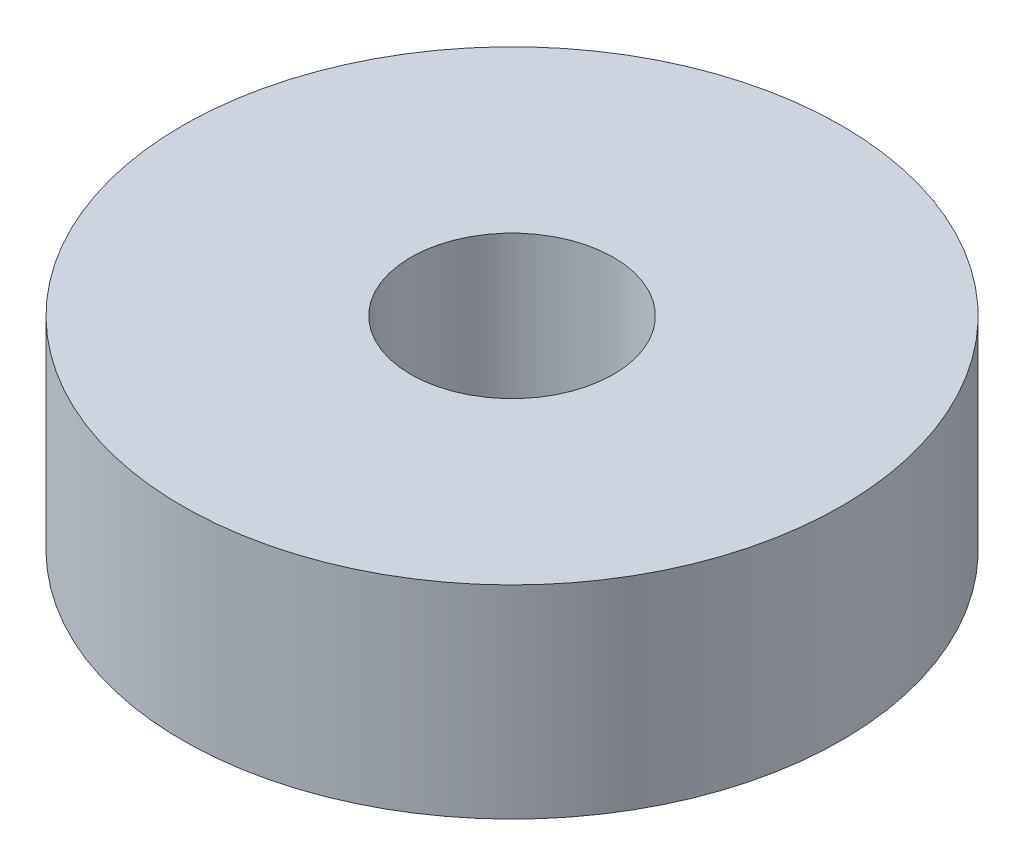
from build123d import *

# Parameters (mm, degrees)
SKETCH_1_W = 4.5
SKETCH_1_H = 4


with BuildPart() as part:
    # 草图1 → 旋转1 (revolve)
    with BuildSketch(Plane.XY, mode=Mode.PRIVATE) as revolve_1_sk:
        with Locations((4.25, -0.346268657)):
            Rectangle(SKETCH_1_W, SKETCH_1_H)
    revolve(revolve_1_sk.sketch.rotate(Axis((0, 0, 0), (0, 1, 0)), 90), axis=Axis((0, 0, 0), (0, 1, 0)))


solid = part.part
